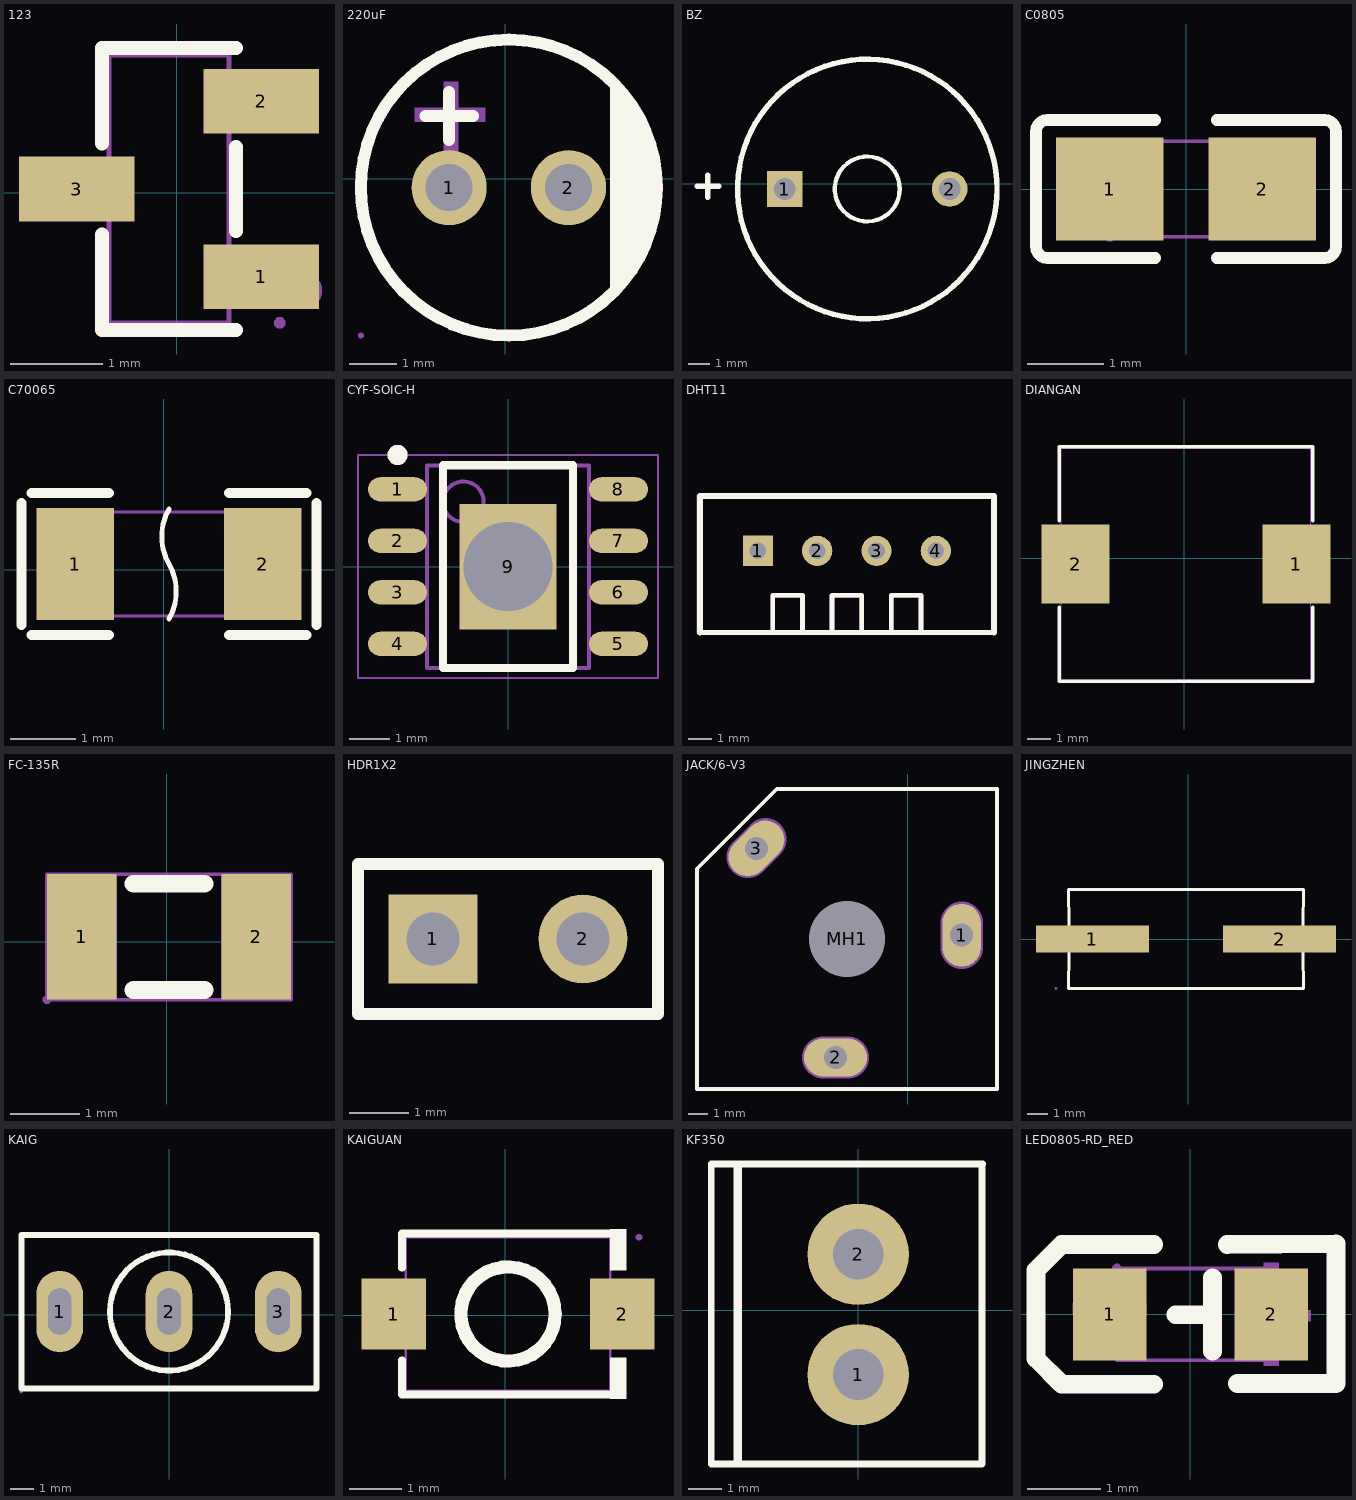
[diagram p0: the footprints below, top view; thin cyan lines are the x and y axes]
# Altium footprint library MISC82341-7.PcbLib: 30 footprints (part 1 of 2)
Each footprint in its own frame and in the unit in brackets; x right, y up, seen from the top. Pads: shape width x height; smd on the part's side, far side on the other; paste and mask are expansions set on the pad; w line width, h text height; cw(c..) or ccw(c..) is an arc to the next point about the centre after c.

## 123 [mm]
pads (3):
  rect 1.25x0.7 smd: 1(0.914,-0.909) 2(0.914,0.99) 3(-1.086,0.04)
Top Overlay:
  lines w0.152: -0.813,-0.454 -0.813,-1.486 0.64,-1.486 ; -0.813,0.535 -0.813,1.567 0.64,1.567 ; 0.64,-0.415 0.64,0.496
Mechanical 6:
  circle w0.2: c1.374,-1.06 r0.1
Mechanical 15:
  region: -1.286,-0.175 -1.286,0.255 -0.986,0.255 -0.986,-0.175
  region: -0.996,-0.175 -0.996,0.255 -0.726,0.255 -0.726,-0.175
  region: 0.814,-1.124 0.814,-0.694 1.114,-0.694 1.114,-1.124
  region: 0.554,-1.124 0.554,-0.694 0.824,-0.694 0.824,-1.124
  region: 0.814,0.775 0.814,1.205 1.114,1.205 1.114,0.775
  region: 0.554,0.775 0.554,1.205 0.824,1.205 0.824,0.775
  region: 1.174,-1.41 1.174,-1.385 1.138,-1.35 1.089,-1.35 1.054,-1.385 1.054,-1.41 1.054,-1.434 1.089,-1.47 1.138,-1.47 1.174,-1.434
  lines w0.051: -0.736,-1.41 0.564,-1.41 0.564,1.49 -0.736,1.49 -0.736,-1.41

## 220uF [mm]
pads (2):
  round 1.6 hole 1: 1(-1.193,-0.185) 2(1.347,-0.185)
Top Overlay:
  circle w0.254: c0.077,-0.185 r3.15
  region: 2.236,2.101 2.395,1.957 2.671,1.627 2.899,1.262 3.074,0.869 3.192,0.456 3.252,0.03 3.252,-0.4 3.192,-0.826 3.074,-1.239 2.899,-1.632 2.671,-1.997 2.395,-2.327 2.236,-2.471
  lines w0.254: -1.701,1.339 -0.685,1.339 ; -1.193,0.831 -1.193,1.847
Mechanical 6:
  region: -1.923,1.515 -0.423,1.515 -0.423,1.215 -1.923,1.215
  region: -1.304,0.567 -1.304,2.067 -1.004,2.067 -1.004,0.567
Mechanical 15:
  region: -3.013,-3.335 -3.013,-3.31 -3.049,-3.275 -3.098,-3.275 -3.133,-3.31 -3.133,-3.335 -3.133,-3.36 -3.098,-3.395 -3.049,-3.395 -3.013,-3.36
  region: 1.647,-0.185 1.647,-0.125 1.601,-0.015 1.517,0.069 1.406,0.115 1.287,0.115 1.177,0.069 1.092,-0.015 1.047,-0.125 1.047,-0.185 1.047,-0.245 1.092,-0.355 1.177,-0.44 1.287,-0.485 1.406,-0.485 1.517,-0.44 1.601,-0.355 1.647,-0.245
  region: -0.893,-0.185 -0.893,-0.125 -0.939,-0.015 -1.023,0.069 -1.134,0.115 -1.253,0.115 -1.363,0.069 -1.448,-0.015 -1.493,-0.125 -1.493,-0.185 -1.493,-0.245 -1.448,-0.355 -1.363,-0.44 -1.253,-0.485 -1.134,-0.485 -1.023,-0.44 -0.939,-0.355 -0.893,-0.245
  lines w0.051: -3.073,-0.185 cw(c0.077,-0.185) 3.227,-0.185 cw(c0.077,-0.185) -3.073,-0.185

## BZ [mm]
pads (2):
  rect 1.65x1.65 hole 1: 1(-13.589,-0.254)
  round 1.65 hole 1: 2(-5.969,-0.254)
Top Overlay:
  circle w0.2: c-9.779,-0.254 r1.5
  circle w0.254: c-9.779,-0.254 r6
  lines w0.254: -17.653,-0.127 -16.637,-0.127 ; -17.145,-0.635 -17.145,0.381

## C0805 [mm]
pads (2):
  rect 1.41x1.35 smd paste-100 mask+0.051: 1(-1,0) 2(1,0)
Top Overlay:
  lines w0.152: -0.401,-0.904 -1.811,-0.904 cw(c-1.811,-0.751) -1.964,-0.751 -1.964,0.751 cw(c-1.811,0.751) -1.811,0.904 -0.401,0.904 ; 0.401,-0.904 1.811,-0.904 ccw(c1.811,-0.751) 1.964,-0.751 1.964,0.751 ccw(c1.811,0.751) 1.811,0.904 0.401,0.904
Top Paste:
  region: -1.675,-0.62 -1.675,0.66 -1.625,0.71 -0.475,0.71 -0.425,0.66 -0.42,0.25 -0.87,0.25 -0.87,-0.2 -0.43,-0.2 -0.425,-0.62 -0.475,-0.67 -1.625,-0.67
  region: 0.475,-0.62 0.475,-0.2 0.92,-0.2 0.92,0.25 0.48,0.25 0.475,0.66 0.525,0.71 1.675,0.71 1.725,0.66 1.725,-0.62 1.675,-0.67 0.525,-0.67
Mechanical 15:
  region: -1,-0.625 -1,0.625 -0.5,0.625 -0.5,-0.625
  region: 1,0.625 1,-0.625 0.5,-0.625 0.5,0.625
  region: -0.94,-0.625 -0.94,-0.6 -0.975,-0.565 -1.025,-0.565 -1.06,-0.6 -1.06,-0.625 -1.06,-0.65 -1.025,-0.685 -0.975,-0.685 -0.94,-0.65
  lines w0.051: -1,-0.625 -1,0.625 1,0.625 1,-0.625 -1,-0.625

## C70065 [mm]
pads (2):
  rect 1.19x1.728 smd: 1(-1.362,0.092) 2(1.528,0.092)
Top Overlay:
  lines w0.076: 0.083,-0.753 ccw(c-0.649,-0.33) 0.083,0.092 cw(c0.815,0.514) 0.083,0.937
  lines w0.152: -2.186,-0.848 -2.186,1.032 ; -2.033,-1.001 -0.843,-1.001 ; -2.033,1.185 -0.843,1.185 ; 1.009,-1.001 2.199,-1.001 ; 1.009,1.185 2.199,1.185 ; 2.352,-0.848 2.352,1.032
Mechanical 15:
  region: -1.457,-0.708 -1.457,-0.683 -1.492,-0.648 -1.542,-0.648 -1.577,-0.683 -1.577,-0.708 -1.577,-0.733 -1.542,-0.768 -1.492,-0.768 -1.457,-0.733
  region: -1.517,-0.708 -1.017,-0.708 -1.017,0.892 -1.517,0.892
  region: 1.183,-0.708 1.683,-0.708 1.683,0.892 1.183,0.892
  lines w0.051: -1.517,-0.708 1.683,-0.708 1.683,0.892 -1.517,0.892 -1.517,-0.708

## CYF-SOIC-H [mm] "SOIC, 8-Leads, Body 4.90x3.90mm, Pitch 1.27mm, Thermal Pad 3.10x2.40mm, IPC Medium Density"
height 1.7
pads (9):
  oval 1.45x0.6 smd: 1(-2.725,1.905) 2(-2.725,0.635) 3(-2.725,-0.635) 4(-2.725,-1.905) 5(2.725,-1.905) 6(2.725,-0.635) 7(2.725,0.635) 8(2.725,1.905)
  rect 2.4x3.1 hole 2.2: 9(0,0)
Top Overlay:
  circle w0.25: c-2.725,2.755 r0.125
  lines w0.2: -1.6,-2.5 -1.6,2.5 1.6,2.5 1.6,-2.5 -1.6,-2.5
Mechanical 13:
  circle w0.1: c-1.1,1.6 r0.5
  lines w0.1: -2,-2.5 -2,2.5 2,2.5 2,-2.5 -2,-2.5
Mechanical 15:
  lines w0.05: -3.7,-2.75 -3.7,2.75 3.7,2.75 3.7,-2.75 -3.7,-2.75
  lines w0.1: -0.5,0 0.5,0 ; 0,-0.5 0,0.5
3D body: height 1.7, standoff 0.15, extent -2,-2.5 2,2.5

## DHT11 [mil]
pads (4):
  rect 51x51 hole 28: 1(-4297.7,2306.22)
  round 51 hole 28: 2(-4197.7,2306.22) 3(-4097.7,2306.22) 4(-3997.7,2306.22)
Top Overlay:
  lines w8: -4396.1,2168.42 -3997.7,2168.42 -3899.3,2168.42 ; -4272.7,2168.42 -4272.7,2231.22 -4222.7,2231.22 -4222.7,2168.42 ; -4172.7,2168.42 -4172.7,2231.22 -4122.7,2231.22 -4122.7,2168.42 ; -4072.7,2168.42 -4072.7,2231.22 -4022.7,2231.22 -4022.7,2168.42
  lines w10: -4395.73,2168.42 -4395.73,2398.73 -3899.67,2398.73 -3899.3,2398.36 -3899.3,2168.42
Mechanical 6:
  region: -4391.01,2172.35 -4391.01,2394 -3904,2394 -3904,2172.35 -4385.1,2172.35 -4385.1,2164.48 -3898.09,2164.48 -3894.55,2168.02 -3894.55,2399.12 -3898.88,2403.45 -4396.52,2403.45 -4400.45,2399.51 -4400.45,2166.84 -4398.09,2164.48 -4385.49,2164.48 -4385.49,2172.35
  region: -4068.96,2172.35 -4076.44,2172.35 -4076.44,2232.19 -4073.68,2234.95 -4021.71,2234.95 -4018.96,2232.19 -4018.96,2172.74 -4026.44,2172.74 -4026.44,2227.07 -4026.83,2227.47 -4068.56,2227.47 -4068.96,2227.07
  region: -4168.95,2172.35 -4176.43,2172.35 -4176.43,2232.19 -4173.68,2234.95 -4121.71,2234.95 -4118.95,2232.19 -4118.95,2172.74 -4126.43,2172.74 -4126.43,2227.07 -4126.83,2227.47 -4168.56,2227.47 -4168.95,2227.07
  region: -4268.96,2172.35 -4276.44,2172.35 -4276.44,2232.19 -4273.68,2234.95 -4221.72,2234.95 -4218.96,2232.19 -4218.96,2172.74 -4226.44,2172.74 -4226.44,2227.07 -4226.83,2227.47 -4268.57,2227.47 -4268.96,2227.07
Mechanical 15:
  region: -4393.37,2167.63 -4393.37,2168.61 -4394.75,2170 -4396.71,2170 -4398.09,2168.61 -4398.09,2167.64 -4398.1,2166.66 -4396.71,2165.27 -4394.75,2165.27 -4393.37,2166.65 -4393.37,2167.63
  region: -4287.86,2300.32 -4307.54,2300.32 -4307.54,2312.13 -4287.86,2312.13
  region: -4187.86,2300.32 -4207.54,2300.32 -4207.54,2312.13 -4187.86,2312.13
  region: -4087.86,2300.32 -4107.54,2300.32 -4107.54,2312.13 -4087.86,2312.13
  region: -3987.86,2300.32 -4007.54,2300.32 -4007.54,2312.13 -3987.86,2312.13
  lines w2: -4395.73,2166.45 -3899.67,2166.45 -3899.67,2398.74 -4395.73,2398.74 -4395.73,2166.45

## DIANGAN [mm]
pads (2):
  rect 2.924x3.42 smd: 1(4.844,-0.241) 2(-4.712,-0.241)
Top Overlay:
  lines w0.152: -5.41,-2.103 -5.41,-5.317 5.542,-5.317 5.542,-2.103 ; -5.41,1.622 -5.41,4.836 5.542,4.836 5.542,1.622
Mechanical 15:
  region: 5.526,4.759 5.526,4.784 5.491,4.819 5.441,4.819 5.406,4.784 5.406,4.759 5.406,4.735 5.441,4.699 5.491,4.699 5.526,4.735
  region: 5.466,-1.741 5.466,1.259 3.466,1.259 3.466,-1.741
  region: -5.334,-1.741 -5.334,1.259 -3.334,1.259 -3.334,-1.741
  lines w0.051: -5.334,-5.241 5.466,-5.241 5.466,4.759 -5.334,4.759 -5.334,-5.241

## FC-135R [mm]
pads (2):
  rect 1x1.8 smd: 1(-1.218,0.071) 2(1.282,0.071)
Top Overlay:
  lines w0.254: -0.476,-0.691 0.54,-0.691 ; -0.476,0.833 0.54,0.833
Mechanical 15:
  region: -1.718,-0.829 -1.718,0.971 -0.718,0.971 -0.718,-0.829
  region: 0.782,-0.829 0.782,0.971 1.782,0.971 1.782,-0.829
  region: -1.658,-0.829 -1.658,-0.804 -1.693,-0.769 -1.743,-0.769 -1.778,-0.804 -1.778,-0.829 -1.778,-0.854 -1.743,-0.889 -1.693,-0.889 -1.658,-0.854
  lines w0.051: -1.718,-0.829 1.782,-0.829 1.782,0.971 -1.718,0.971 -1.718,-0.829

## HDR1X2 [mm]
pads (2):
  rect 1.5x1.5 hole 0.9: 1(-70.739,15.748)
  round 1.5 hole 0.9: 2(-68.199,15.748)
Top Overlay:
  lines w0.2: -72.009,14.478 -66.929,14.478 -66.929,17.018 -72.009,17.018 -72.009,14.478

## JACK/6-V3 [mm]
pads (4):
  oval 2x3.3 hole 1.2: 1(2.825,-37.773)
  oval 3.3x2 hole 1.2: 2(-3.775,-44.173)
  oval 2x3.3 hole 1.2 rot 135: 3(-7.913,-33.235)
  round 3.7 hole 4: MH1(-3.175,-37.973)
Top Overlay:
  lines w0.2: -11.025,-45.823 -11.025,-34.298 -6.85,-30.123 4.675,-30.123 4.675,-45.823 -11.025,-45.823
Mechanical 1:
  lines w1.2: -8.36,-33.678 -7.441,-32.759 ; -4.425,-44.173 -3.125,-44.173 ; 2.825,-38.423 2.825,-37.123
Mechanical 2:
  lines w2.216: -8.36,-33.678 -7.441,-32.759 ; -4.425,-44.173 -3.125,-44.173 ; 2.825,-38.423 2.825,-37.123

## JINGZHEN [mm]
pads (2):
  rect 5.5x1.3 smd: 1(-4.665,0.013) 2(4.441,0.013)
Top Overlay:
  lines w0.152: -5.827,-2.4 -5.812,-0.649 -5.827,-2.4 ; -5.827,-2.4 5.603,-2.4 ; -5.827,-2.4 5.603,-2.4 ; -5.827,2.426 5.603,2.426 ; -5.827,2.426 -5.812,0.676 -5.827,2.426 ; -5.827,2.426 5.603,2.426 ; 5.603,-2.4 5.588,-0.649 5.603,-2.4 ; 5.603,2.426 5.588,0.676 5.603,2.426
Mechanical 15:
  region: -6.393,-2.387 -6.393,-2.362 -6.428,-2.327 -6.477,-2.327 -6.512,-2.362 -6.512,-2.387 -6.512,-2.412 -6.477,-2.447 -6.428,-2.447 -6.393,-2.412
  region: -1.952,-0.387 -6.452,-0.387 -6.452,0.413 -1.952,0.413
  region: 6.228,-0.387 1.728,-0.387 1.728,0.413 6.228,0.413
  lines w0.051: -5.812,-2.387 5.588,-2.387 5.588,2.413 -5.812,2.413 -5.812,-2.387

## KAIG [mm]
pads (3):
  oval 2x3.5 hole 1 slot 2 at 90 deg paste+0 mask+0.05: 1(-4.709,0.135) 2(-0.009,0.135) 3(4.691,0.135)
Top Overlay:
  circle w0.254: c-0.009,0.135 r2.54
  lines w0.254: -6.359,-3.165 6.341,-3.165 6.341,3.435 -6.359,3.435 -6.359,-3.165
Mechanical 15:
  region: -6.299,-3.315 -6.299,-3.29 -6.334,-3.255 -6.384,-3.255 -6.419,-3.29 -6.419,-3.315 -6.419,-3.34 -6.384,-3.375 -6.334,-3.375 -6.299,-3.34
  region: -4.329,1.135 -4.329,-0.865 -5.089,-0.865 -5.089,1.135
  region: 0.371,1.135 0.371,-0.865 -0.389,-0.865 -0.389,1.135
  region: 5.071,1.135 5.071,-0.865 4.311,-0.865 4.311,1.135

## KAIGUAN [mm]
pads (2):
  rect 1.23x1.36 smd: 1(-2.13,0.027) 2(2.24,0.027)
Top Overlay:
  circle w0.254: c0.055,0.027 r0.9
  region: 2.005,-1.59 2.005,-0.805 2.31,-0.805 2.31,-1.59
  region: 2.005,1.644 2.005,0.859 2.31,0.859 2.31,1.644
  lines w0.152: -1.971,-0.856 -1.971,-1.514 2.081,-1.514 ; -1.971,0.91 -1.971,1.568 2.081,1.568
Mechanical 15:
  region: 2.615,1.492 2.615,1.517 2.58,1.552 2.531,1.552 2.495,1.517 2.495,1.492 2.495,1.467 2.531,1.432 2.58,1.432 2.615,1.467
  region: 2.555,0.677 2.555,-0.623 1.655,-0.623 1.655,0.677
  region: -2.445,0.677 -2.445,-0.623 -1.545,-0.623 -1.545,0.677
  lines w0.051: -1.895,-1.438 2.005,-1.438 2.005,1.492 -1.895,1.492 -1.895,-1.438

## KF350 [mm]
pads (2):
  round 3 hole 1.5: 1(0,-1.905) 2(0,1.651)
Top Overlay:
  lines w0.2: -4.343,4.318 -4.343,-4.547 3.658,-4.547 3.658,4.318 ; -4.318,4.318 3.683,4.318
  lines w0.254: -3.556,-4.445 -3.556,4.191

## LED0805-RD_RED [mm]
pads (2):
  rect 1x1.25 smd: 1(-1.1,0) 2(1.1,0)
Top Overlay:
  lines w0.254: -0.5,-0.95 -1.75,-0.95 ; -0.5,0.95 -1.75,0.95 ; -0.2,-0.005 0.3,-0.005 ; 0.3,-0.5 0.3,0.5 ; 0.5,0.95 1.98,0.96 1.98,-0.94 0.64,-0.94 ; -1.75,-0.95 -2.1,-0.6 -2.1,0.6 -1.75,0.95 ; -1.75,-0.95 -1.75,-0.95 ; -1.75,0.95 -1.75,0.95
Mechanical 6:
  region: -1.6,0 -0.6,0 -0.6,0.15 -1.6,0.15
  region: 0.635,-0.094 1.635,-0.094 1.635,0.056 0.635,0.056
  region: 1,0.7 1.2,0.7 1.2,-0.7 1,-0.7
Mechanical 15:
  region: -0.65,-0.625 -1,-0.625 -1,0.625 -0.65,0.625
  region: 1,-0.625 0.65,-0.625 0.65,0.625 1,0.625
  region: -0.94,0.625 -0.94,0.65 -0.975,0.685 -1.025,0.685 -1.06,0.65 -1.06,0.625 -1.06,0.6 -1.025,0.565 -0.975,0.565 -0.94,0.6
  lines w0.051: -1,-0.625 1,-0.625 1,0.625 -1,0.625 -1,-0.625